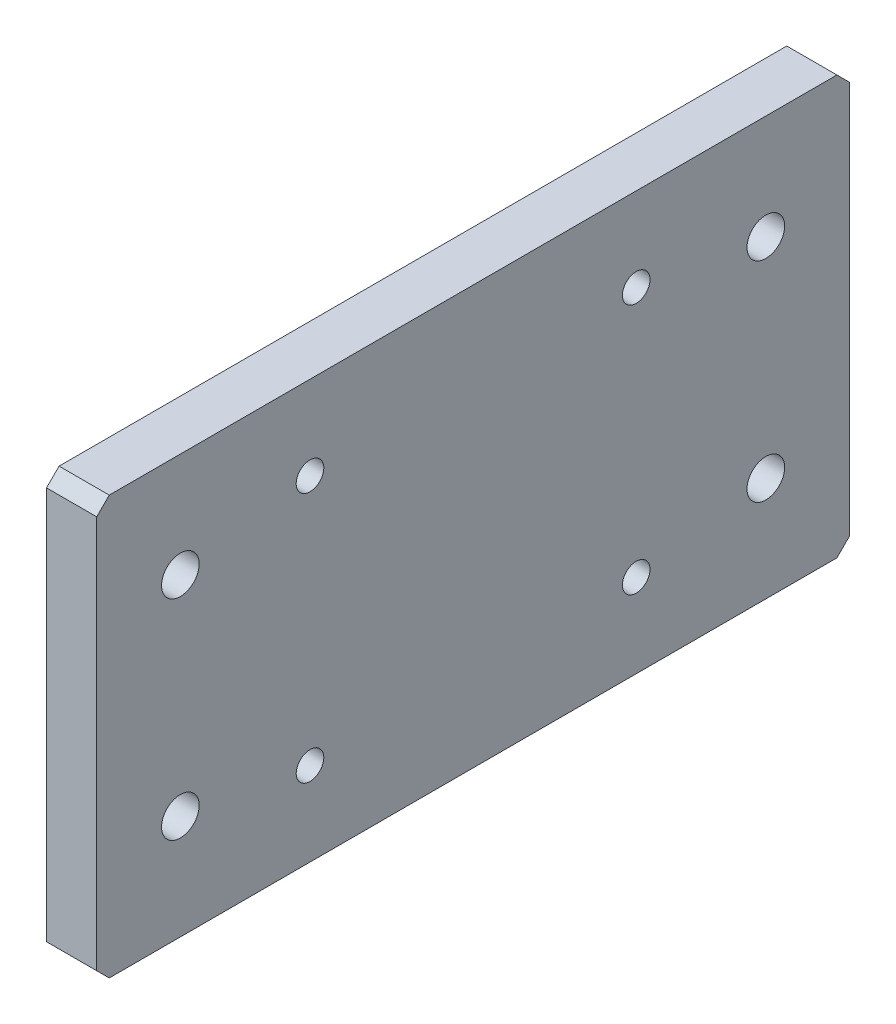
from build123d import *

# Parameters (mm, degrees)
SKETCH_1_W                = 180
SKETCH_1_H                = 100
EXTRUDE_1_DEPTH           = 12
HOLE_WIZARD_1_D           = 6.6
HOLE_WIZARD_1_CBORE_D     = 11
HOLE_WIZARD_1_CBORE_DEPTH = 6.8
HOLE_WIZARD_9_0_9_1_D     = 9
CHAMFER_1_SIZE            = 3


with BuildPart() as part:
    # 草图1 → 凸台-拉伸1 (new body)
    with BuildSketch(Plane(origin=(0, 0, 0), x_dir=(0, 0, -1), z_dir=(1, 0, 0))):
        Rectangle(SKETCH_1_W, SKETCH_1_H)
    extrude(amount=EXTRUDE_1_DEPTH)

    # 打孔尺寸(%根据)内六角圆柱头螺钉的类型1 (through all)
    with Locations(Plane.ZY):
        with Locations((-39, 30), (-39, -30), (39, 30), (39, -30)):
            CounterBoreHole(HOLE_WIZARD_1_D / 2, HOLE_WIZARD_1_CBORE_D / 2, HOLE_WIZARD_1_CBORE_DEPTH)

    # Ø9.0 (9) 直径孔1 (through all)
    with Locations(Plane.ZY):
        with Locations((-70, 25), (-70, -25), (70, 25), (70, -25)):
            Hole(HOLE_WIZARD_9_0_9_1_D / 2)

    # 倒角1
    chamfer_1_edges = [part.edges().sort_by_distance(p)[0] for p in [
        (6, -50, -90),
        (6, -50, 90),
        (6, 50, 90),
        (6, 50, -90),
    ]]
    chamfer(chamfer_1_edges, length=CHAMFER_1_SIZE)


solid = part.part
